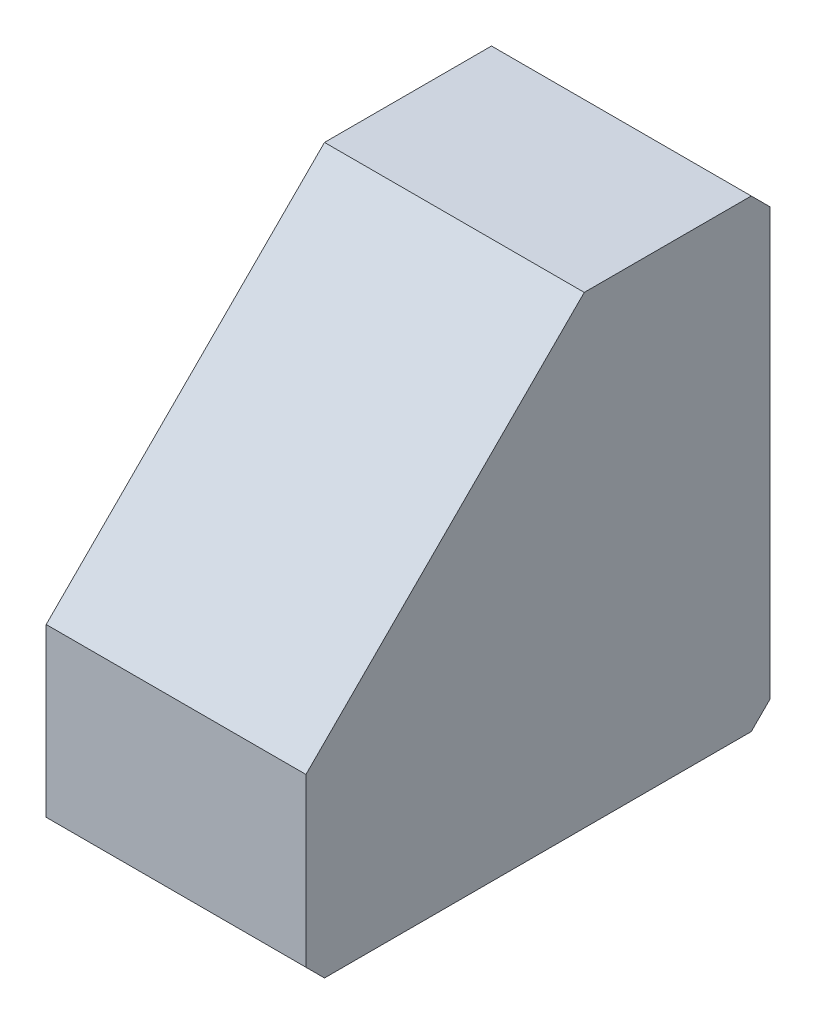
from build123d import *

# Parameters (mm, degrees)
BOSS_EXTRUDE1_DEPTH   = 7
M6_TAPPED_HOLE1_D     = 5
M6_TAPPED_HOLE1_DEPTH = 15
M6_TAPPED_HOLE1_TIP   = 1.502151548
M6_TAPPED_HOLE2_D     = 5
M6_TAPPED_HOLE2_DEPTH = 15
M6_TAPPED_HOLE2_TIP   = 1.502151548
CHAMFER1_SIZE         = 1


with BuildPart() as part:
    # Sketch1 → Boss-Extrude1 (new, symmetric)
    with BuildSketch(Plane(origin=(0, 0, 0), x_dir=(0, 0, -1), z_dir=(1, 0, 0))):
        Polygon((0, 0), (0, 25), (-10, 25), (-25, 10), (-25, 0), align=None)
    extrude(amount=BOSS_EXTRUDE1_DEPTH, both=True)

    # M6 Tapped Hole1
    with Locations(Plane(origin=(0, 0, 0), x_dir=(-1, 0, 0), z_dir=(0, -1, 0))):
        with Locations((0, -15)):
            Hole(M6_TAPPED_HOLE1_D / 2, depth=M6_TAPPED_HOLE1_DEPTH)
            with Locations((0, 0, -(M6_TAPPED_HOLE1_DEPTH + M6_TAPPED_HOLE1_TIP / 2))):  # 118° drill point
                Cone(0, M6_TAPPED_HOLE1_D / 2, M6_TAPPED_HOLE1_TIP, mode=Mode.SUBTRACT)

    # M6 Tapped Hole2
    with Locations(Plane(origin=(0, 0, 0), x_dir=(-1, 0, 0), z_dir=(0, 0, -1))):
        with Locations((0, 15)):
            Hole(M6_TAPPED_HOLE2_D / 2, depth=M6_TAPPED_HOLE2_DEPTH)
            with Locations((0, 0, -(M6_TAPPED_HOLE2_DEPTH + M6_TAPPED_HOLE2_TIP / 2))):  # 118° drill point
                Cone(0, M6_TAPPED_HOLE2_D / 2, M6_TAPPED_HOLE2_TIP, mode=Mode.SUBTRACT)

    # Chamfer1
    chamfer1_edges = [part.edges().sort_by_distance(p)[0] for p in [
        (0, 0, 25),
        (0, 25, 0),
        (0, 0, 0),
    ]]
    chamfer(chamfer1_edges, length=CHAMFER1_SIZE)


solid = part.part
